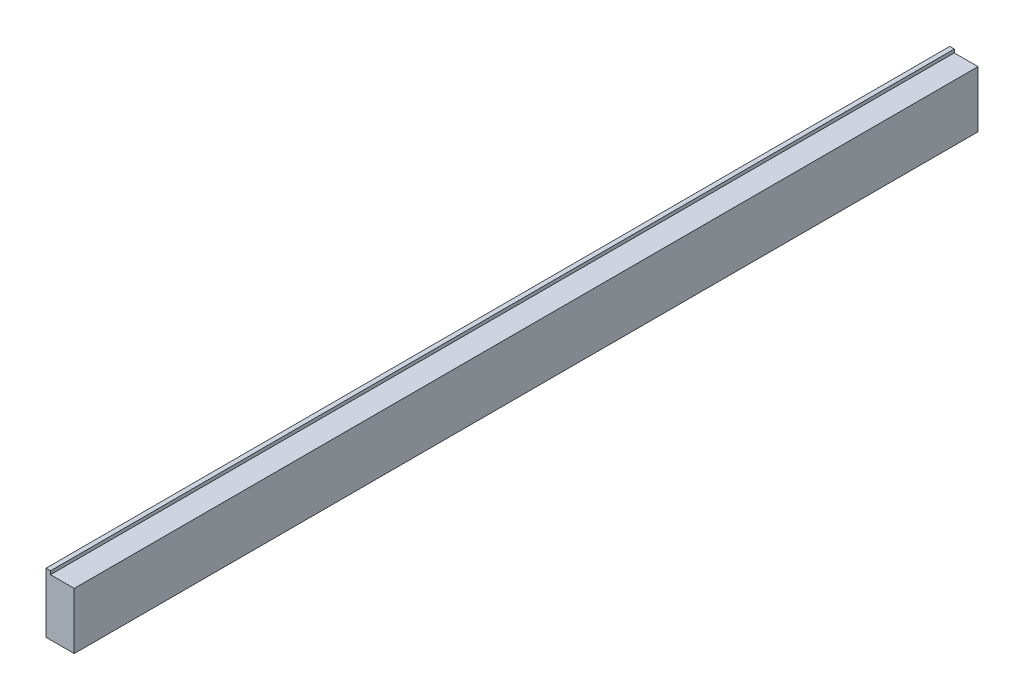
from build123d import *

# Parameters (mm, degrees)
EXTRUDE_1_DEPTH = 800


with BuildPart() as part:
    # 草图1 → 凸台-拉伸1 (new body)
    with BuildSketch(Plane.XY):
        Polygon((-10, -12.5), (-14, -12.5), (-14, -65.5), (11, -65.5), (11, -15.5), (-10, -15.5), align=None)
    extrude(amount=-EXTRUDE_1_DEPTH)


solid = part.part
